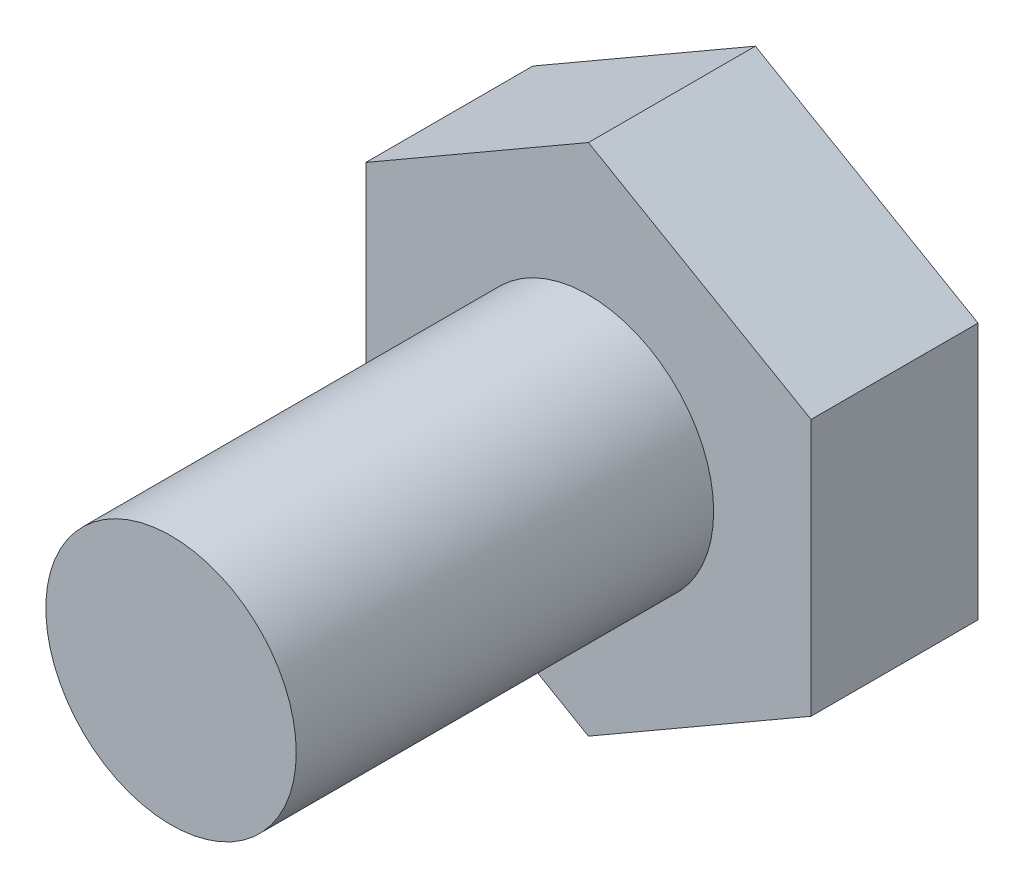
SolidWorks part; units mm, degrees
ref_plane "Front Plane" through (0, 0, 0) normal (0, 0, 1) x (1, 0, 0)
ref_plane "Top Plane" through (0, 0, 0) normal (0, 1, 0) x (1, 0, 0)
ref_plane "Right Plane" through (0, 0, 0) normal (1, 0, 0) x (0, 0, -1)
sketch "Sketch2" plane through (0, 0, 0) normal (0, 0, 1) x (1, 0, 0)
  line L1 (0, 9.2376) -> (-8, 4.6188)
  line L2 (-8, 4.6188) -> (-8, -4.6188)
  line L3 (-8, -4.6188) -> (0, -9.2376)
  line L4 (0, -9.2376) -> (8, -4.6188)
  line L5 (8, -4.6188) -> (8, 4.6188)
  line L6 (8, 4.6188) -> (0, 9.2376)
  circle A0 centre (0, 0) radius 8 construction
extrude "Boss-Extrude2" add sketch "Sketch2" along normal blind 6
sketch "Sketch3" plane through (0, 0, 6) normal (0, 0, 1) x (1, 0, 0)
  circle A0 centre (0, 0) radius 4.5
extrude "Boss-Extrude3" add sketch "Sketch3" along normal blind 15
